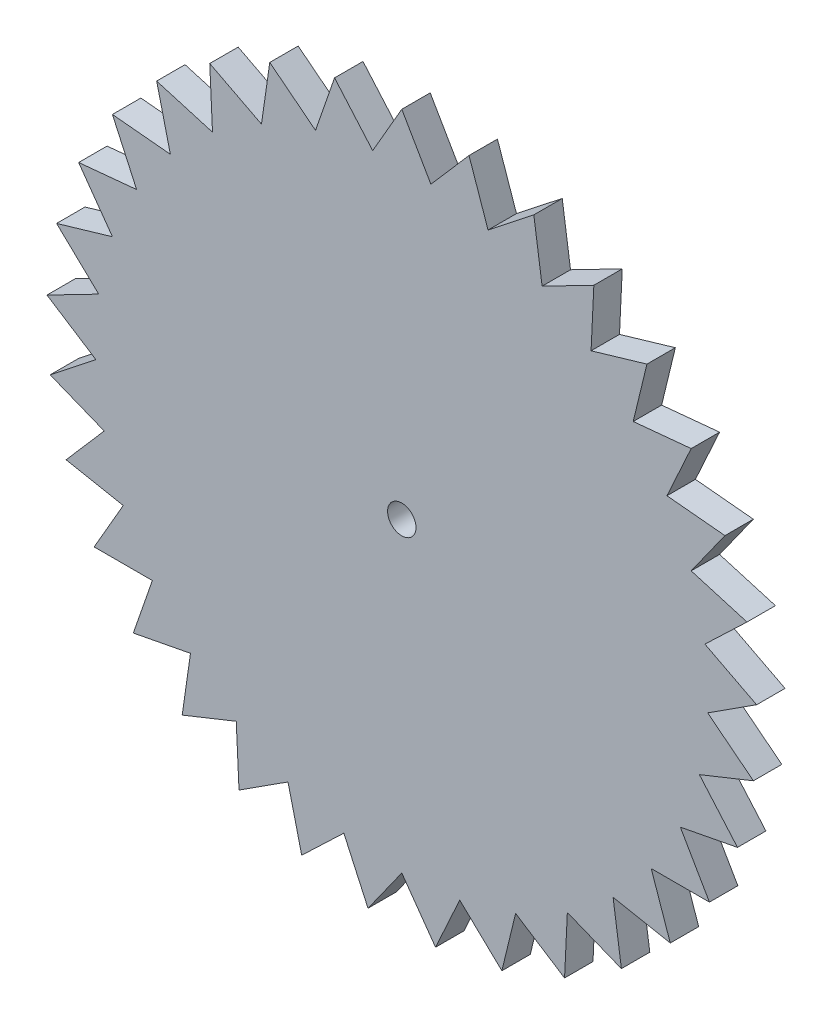
from build123d import *

# Parameters (mm, degrees)
SKETCH_1_R      = 5
EXTRUDE_4_DEPTH = 10


with BuildPart() as part:
    # 草图1 → 凸台-拉伸4 (new body)
    with BuildSketch(Plane.XY):
        Polygon((0, 125), (-10.24210316, 107.26015695), (-23.656405545, 122.741087158), (-30.356133186, 103.383495415), (-46.457806958, 116.045991627), (-49.373013467, 95.770284992), (-67.580102182, 105.156691604), (-66.605424401, 84.695686942), (-86.259876435, 90.466754763), (-81.430541758, 70.559966093), (-101.821994006, 72.507113696), (-93.312547172, 53.874024228), (-113.703999419, 51.926876625), (-101.821994006, 35.24093476), (-121.47644604, 29.469866939), (-106.651328683, 15.33414609), (-124.858417398, 5.947739478), (-107.626006464, -5.126858572), (-123.727680235, -17.789354784), (-104.710799954, -25.402565207), (-118.125102339, -40.883495415), (-98.011072313, -44.76015695), (-108.253175473, -62.5), (-87.768969153, -62.5), (-94.468696794, -81.857591743), (-74.354666768, -77.980930207), (-77.269873278, -98.256636843), (-58.252992997, -90.64342642), (-57.278315216, -111.104431082), (-40.045904282, -100.029833032), (-35.216569605, -119.936621702), (-20.391452248, -105.800900853), (-11.882005413, -124.433990322), (0, -107.748048456), (11.882005413, -124.433990322), (20.391452248, -105.800900853), (35.216569605, -119.936621702), (40.045904282, -100.029833032), (57.278315216, -111.104431082), (58.252992997, -90.64342642), (77.269873278, -98.256636843), (74.354666768, -77.980930207), (94.468696794, -81.857591743), (87.768969153, -62.5), (108.253175473, -62.5), (98.011072313, -44.76015695), (118.125102339, -40.883495415), (104.710799954, -25.402565207), (123.727680235, -17.789354784), (107.626006464, -5.126858572), (124.858417398, 5.947739478), (106.651328683, 15.33414609), (121.47644604, 29.469866939), (101.821994006, 35.24093476), (113.703999419, 51.926876625), (93.312547172, 53.874024228), (101.821994006, 72.507113696), (81.430541758, 70.559966093), (86.259876435, 90.466754763), (66.605424401, 84.695686942), (67.580102182, 105.156691604), (49.373013467, 95.770284992), (46.457806958, 116.045991627), (30.356133186, 103.383495415), (23.656405545, 122.741087158), (10.24210316, 107.26015695), align=None)
        Circle(SKETCH_1_R, mode=Mode.SUBTRACT)
    extrude(amount=EXTRUDE_4_DEPTH)


solid = part.part
